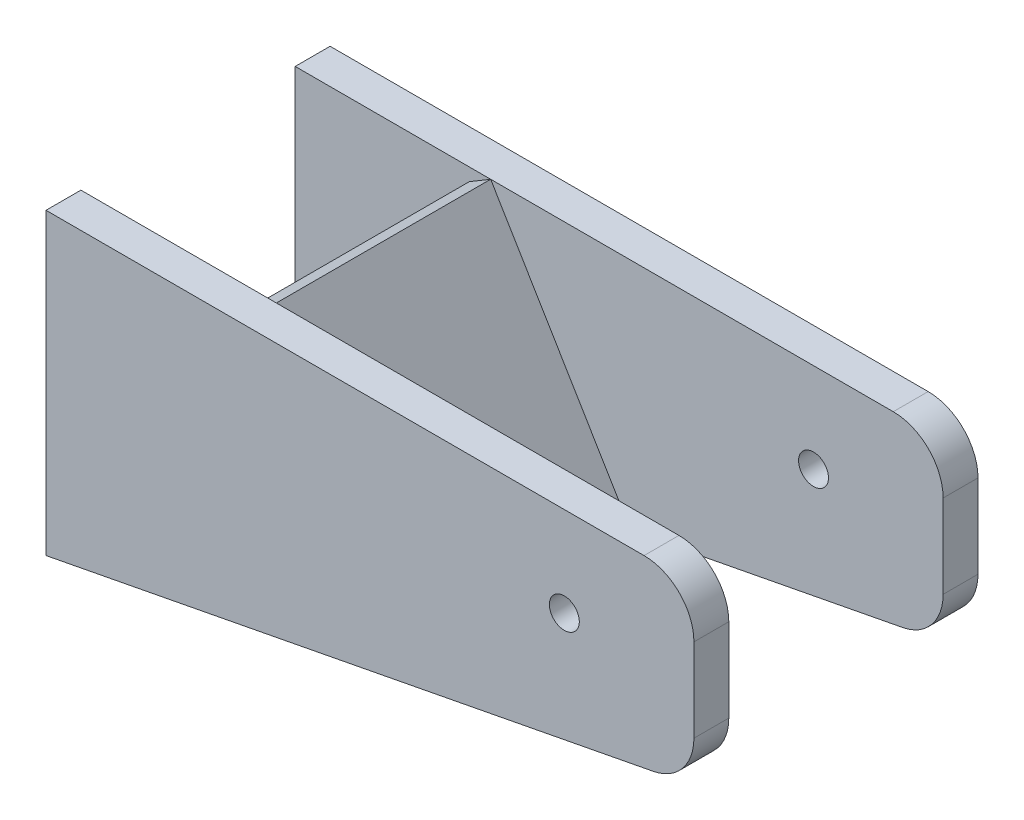
from build123d import *

# Parameters (mm, degrees)
SKETCH_1_W             = 7
SKETCH_1_H             = 60
EXTRUDE_1_DEPTH        = 130
SKETCH_2_R             = 3
CUT_EXTRUDE_1_DEPTH    = 826.099387953
FILLET_1_R             = 10
PATTERN_LINEAR_2_COUNT = 2
PATTERN_LINEAR_2_PITCH = 50
EXTRUDE_2_REACH        = 828.583


with BuildPart() as part:
    # 草图1 → 凸台-拉伸1 (new body)
    with BuildSketch(Plane(origin=(686, 0, 0), x_dir=(0, 0, -1), z_dir=(1, 0, 0))):
        with Locations((1691.5, 92)):
            Rectangle(SKETCH_1_W, SKETCH_1_H)
    extrude(amount=EXTRUDE_1_DEPTH)

    # 草图2 → 切除-拉伸1 (cut, through all)
    with BuildSketch(Plane(origin=(0, 0, -1695), x_dir=(-1, 0, 0), z_dir=(0, 0, -1))):
        with Locations((-790, 104)):
            Circle(SKETCH_2_R)
        Polygon((-816, 87), (-686, 62), (-816, 62), align=None)
    extrude(amount=-CUT_EXTRUDE_1_DEPTH, mode=Mode.SUBTRACT)

    # 圆角1
    fillet_1_edges = [part.edges().sort_by_distance(p)[0] for p in [
        (816, 122, -1691.5),
        (816, 87, -1691.5),
    ]]
    fillet(fillet_1_edges, radius=FILLET_1_R)


with BuildPart() as pattern_linear_2_1:
    # 阵列(线性)2: pattern copy
    add(part.part.moved(Location(Vector(0, 0, 1) * (1 * PATTERN_LINEAR_2_PITCH))))


with BuildPart() as body_3:

    # 草图3 → 凸台-拉伸2 (new, up to next)
    with BuildSketch(Plane.XY.offset(-1688), mode=Mode.PRIVATE) as extrude_2_sk1:
        Polygon((720.928933922, 119.43337756), (748.135131786, 73.949063805), (752.426104782, 76.515686245), (725.219906917, 122), align=None)
    extrude_2_tool1 = extrude(extrude_2_sk1.sketch, amount=EXTRUDE_2_REACH, mode=Mode.PRIVATE) - pattern_linear_2_1.part
    add(extrude_2_tool1.solids().sort_by_distance((736.677519, 97.974532, -1688))[0])


solid = Compound([part.part, pattern_linear_2_1.part, body_3.part])
